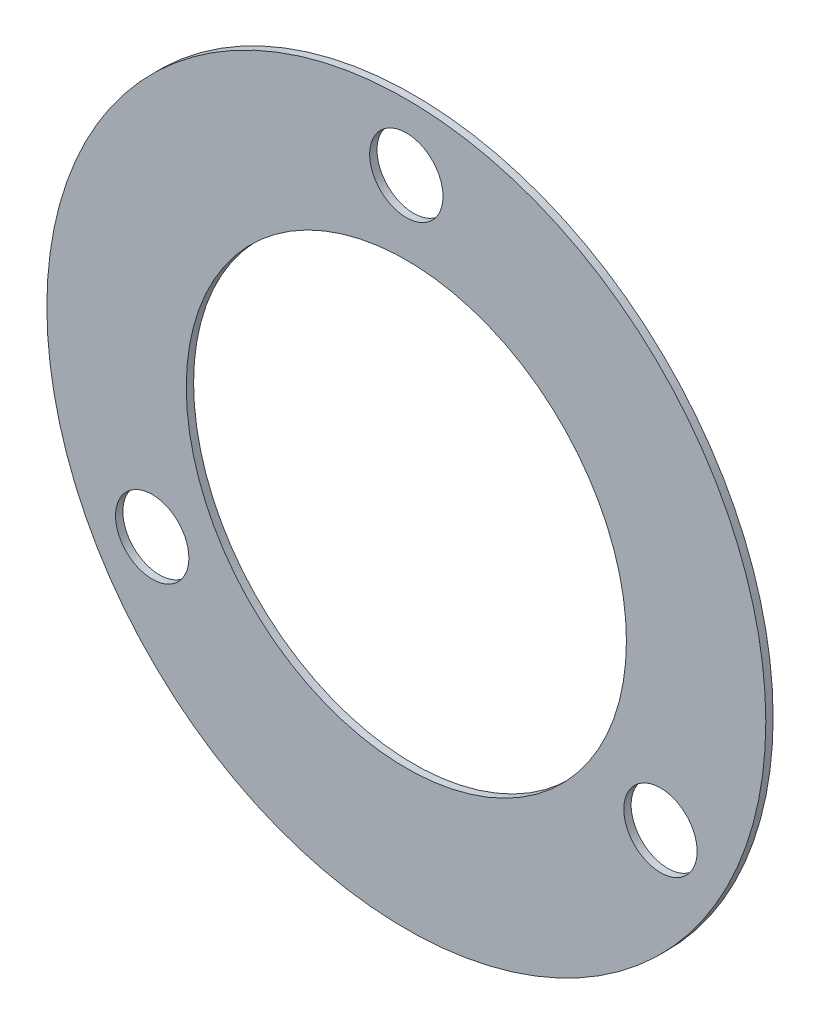
from build123d import *

# Parameters (mm, degrees)
SKETCH1_R           = 24.5
SKETCH1_R_2         = 15
BOSS_EXTRUDE1_DEPTH = 0.5
SKETCH2_R           = 2.5
CUT_EXTRUDE1_DEPTH  = 0.5


with BuildPart() as part:
    # Sketch1 → Boss-Extrude1 (new body)
    with BuildSketch(Plane.XY):
        Circle(SKETCH1_R)
        Circle(SKETCH1_R_2, mode=Mode.SUBTRACT)
    extrude(amount=BOSS_EXTRUDE1_DEPTH)

    # Sketch2 → Cut-Extrude1 (cut)
    with BuildSketch(Plane.XY.offset(0.5)):
        with Locations((0, 20)):
            Circle(SKETCH2_R)
        with Locations((17.320508076, -10)):
            Circle(SKETCH2_R)
        with Locations((-17.320508076, -10)):
            Circle(SKETCH2_R)
    extrude(amount=-CUT_EXTRUDE1_DEPTH, mode=Mode.SUBTRACT)


solid = part.part
